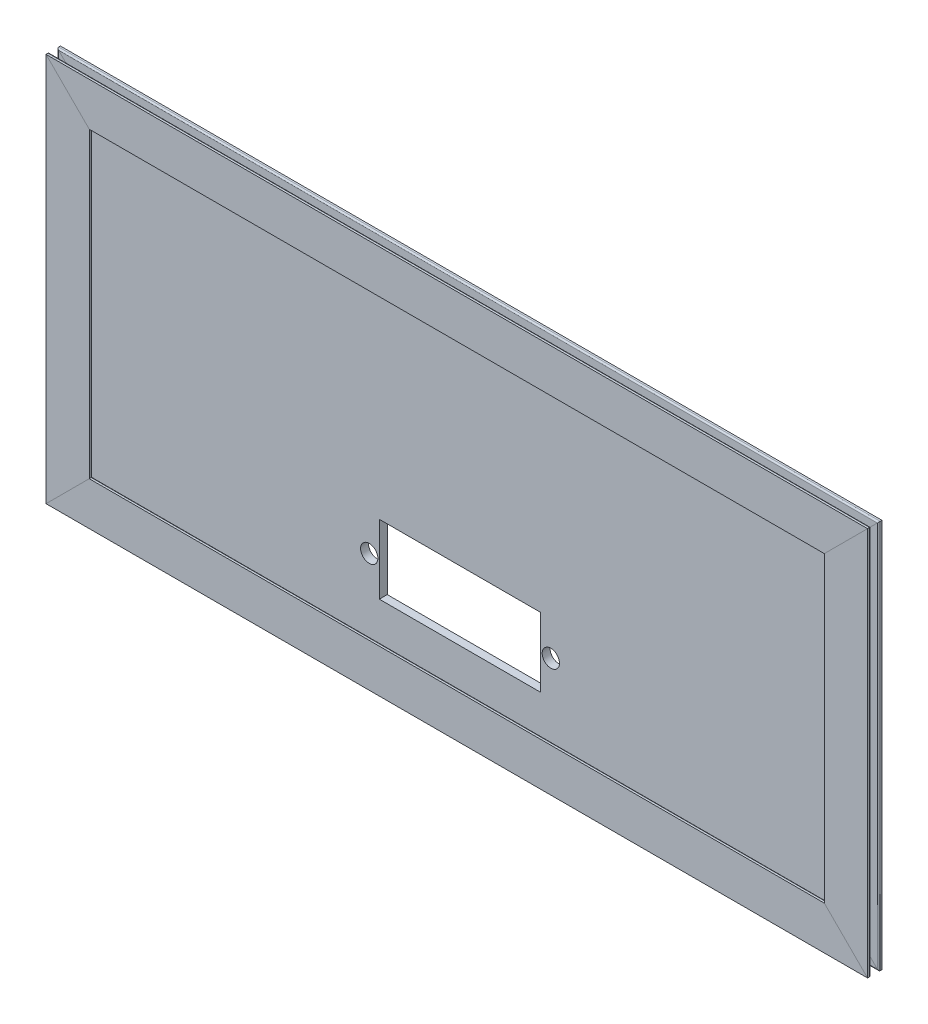
SolidWorks part; units mm, degrees
ref_plane "Front Plane" through (0, 0, 0) normal (0, 0, 1) x (1, 0, 0)
ref_plane "Top Plane" through (0, 0, 0) normal (0, 1, 0) x (1, 0, 0)
ref_plane "Right Plane" through (0, 0, 0) normal (1, 0, 0) x (0, 0, -1)
sketch "Sketch 1" plane through (0, 0, 0) normal (0, 0, 1) x (1, 0, 0)
  line L1 (-270, -120) -> (270, -120)
  line L2 (-270, -120) -> (-270, 120)
  line L3 (-270, 120) -> (270, 120)
  line L4 (270, -120) -> (270, 120)
  line L5 (-270, -120) -> (270, 120) construction
  line L6 (-270, 120) -> (270, -120) construction
  point P0 (0, 0)
  dimension "D1" = 540
  dimension "D2" = 240
other "Aluminium profile 20 X 20 X 2(1)"
ref_plane "Plane1" through (-270, 120, 0) normal (1, 0, 0) x (0, 1, 0)
sketch "Sketch1" plane through (-270, 120, 0) normal (1, 0, 0) x (0, 1, 0)
  line L0 (-3.1, -2.2) -> (3.1, -2.2)
  line L1 (3.1, -2.2) -> (3.1, 2.2)
  line L2 (3.1, 2.2) -> (-3.1, 2.2)
  line L3 (-3.1, 2.2) -> (-3.1, -2.2)
  line L4 (4.5, 2.75) -> (14, 2.75)
  line L5 (4.5, -2.75) -> (4.5, 2.75)
  line L6 (14, -2.75) -> (4.5, -2.75)
  line L7 (15, -5) -> (15, -3.75)
  line L8 (-15, -5) -> (15, -5)
  line L9 (-15, -3.75) -> (-15, -5)
  line L10 (-4.5, -2.75) -> (-14, -2.75)
  line L11 (-4.5, 2.75) -> (-4.5, -2.75)
  line L12 (-14, 2.75) -> (-4.5, 2.75)
  line L13 (-15, 5) -> (-15, 3.75)
  line L14 (15, 5) -> (-15, 5)
  line L15 (15, 3.75) -> (15, 5)
  arc A0 (15, -3.75) -> (14, -2.75) centre (14, -3.75) ccw
  arc A1 (-14, -2.75) -> (-15, -3.75) centre (-14, -3.75) ccw
  arc A2 (-15, 3.75) -> (-14, 2.75) centre (-14, 3.75) ccw
  arc A3 (14, 2.75) -> (15, 3.75) centre (14, 3.75) ccw
  point P24 (0, 0)
sketch "Sketch3" plane through (0, 0, -2.75) normal (0, 0, 1) x (1, 0, 0)
  line L1 (-256, 106) -> (256, 106)
  line L2 (-256, 106) -> (-256, -106)
  line L3 (-256, -106) -> (256, -106)
  line L4 (256, 106) -> (256, -106)
extrude "Boss-Extrude1" add sketch "Sketch3" along normal up to surface (5.5 mm away) separate body up to face at (0, -110.75, 2.75)
sketch "Sketch4" plane through (0, 0, -2.75) normal (0, 0, -1) x (-1, 0, 0)
  line L0 (255, -105) -> (-255, -105) construction
  line L1 (56, -79) -> (-56, -79)
  line L2 (56, -79) -> (56, -31)
  line L3 (56, -31) -> (-56, -31)
  line L4 (-56, -79) -> (-56, -31)
  line L5 (56, -79) -> (-56, -31) construction
  line L6 (56, -31) -> (-56, -79) construction
  line L7 (-63, -55) -> (63, -55) construction
  line L8 (0, 0) -> (0, -55) construction
  circle A0 centre (-63, -55) radius 6
  circle A1 centre (63, -55) radius 6
  point P0 (0, -55)
  point P15 (0, -55)
  dimension "D5" = 12
  dimension "D1" = 50
  dimension "D2" = 112
  dimension "D3" = 48
  dimension "D4" = 126
extrude "Cut-Extrude1" cut sketch "Sketch4" against normal through all
